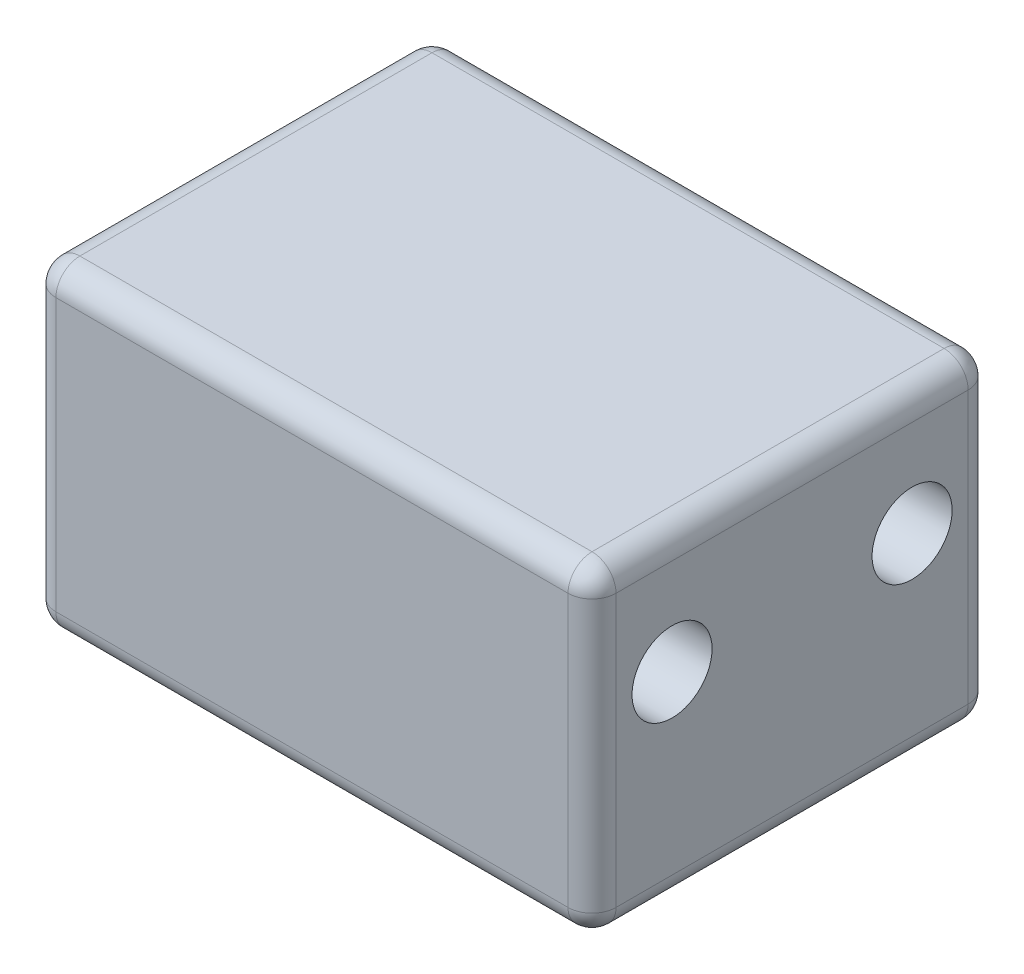
SolidWorks part; units mm, degrees
material "Beech"
ref_plane "Front Plane" through (0, 0, 0) normal (0, 0, 1) x (1, 0, 0)
ref_plane "Top Plane" through (0, 0, 0) normal (0, 1, 0) x (1, 0, 0)
ref_plane "Right Plane" through (0, 0, 0) normal (1, 0, 0) x (0, 0, -1)
sketch "Sketch1" plane through (0, 0, 0) normal (0, 1, 0) x (1, 0, 0)
  line L1 (0, 0) -> (70, 0)
  line L2 (0, 0) -> (0, 50)
  line L3 (0, 50) -> (70, 50)
  line L4 (70, 0) -> (70, 50)
  dimension "D1" = 70
  dimension "D2" = 50
extrude "Boss-Extrude1" add sketch "Sketch1" along normal blind 40
sketch "Sketch2" plane through (70, 0, 0) normal (1, 0, 0) x (0, 0, -1)
  line L0 (25, 40) -> (25, 0) construction
  line L1 (0, 40) -> (50, 40) construction
  line L2 (0, 0) -> (50, 0) construction
  circle A0 centre (40, 25) radius 5
  circle A1 centre (10, 25) radius 5
  dimension "D1" = 15
  dimension "D2" = 10
  dimension "D3" = 30
extrude "Cut-Extrude1" cut sketch "Sketch2" against normal through all
sketch "Sketch3" plane through (0, 0, 0) normal (0, -1, 0) x (1, 0, 0)
  line L0 (35, 0) -> (35, -50) construction
  line L1 (0, 0) -> (70, 0) construction
  line L2 (70, -50) -> (0, -50) construction
  line L3 (0, -25) -> (70, -25) construction
  line L4 (0, -50) -> (0, 0) construction
  line L5 (70, 0) -> (70, -50) construction
  circle A0 centre (60, -25) radius 6
  dimension "D1" = 10
  dimension "D2" = 12
extrude "Cut-Extrude2" cut sketch "Sketch3" against normal blind 35
sketch "Sketch4" plane through (0, 0, 0) normal (0, -1, 0) x (1, 0, 0)
  line L0 (0, -25) -> (70, -25) construction
  line L1 (0, -50) -> (0, 0) construction
  line L2 (70, 0) -> (70, -50) construction
  circle A0 centre (15, -25) radius 10.5
  circle A1 centre (60, -25) radius 6 construction
  dimension "D1" = 21
  dimension "D2" = 45
extrude "Cut-Extrude3" cut sketch "Sketch4" against normal blind 7
fillet "Fillet1" radius 3 12 edges at (35, 40, -50) (70, 40, -25) (35, 40, 0) (0, 40, -25) (0, 20, 0) (70, 20, -50) (0, 20, -50) (70, 20, 0) (70, 0, -25) (35, 0, -50) (0, 0, -25) (35, 0, 0)
